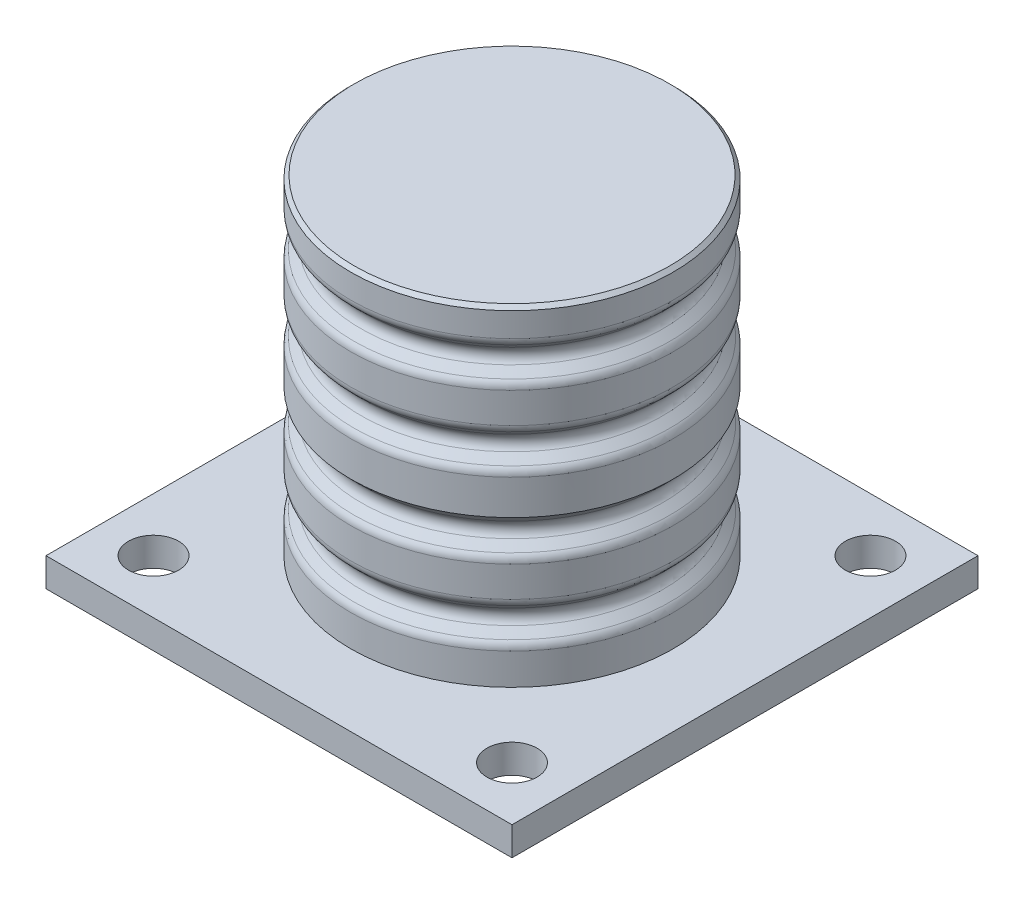
from build123d import *

# Parameters (mm, degrees)
SKETCH2_W           = 130
SKETCH2_H           = 130
SKETCH2_R           = 7
BOSS_EXTRUDE1_DEPTH = 8
SKETCH3_R           = 45
BOSS_EXTRUDE2_DEPTH = 100
CHAMFER1_SIZE       = 1
FILLET1_R           = 3


with BuildPart() as part:
    # Sketch2 → Boss-Extrude1 (new body)
    with BuildSketch(Plane(origin=(0, 0, 0), x_dir=(1, 0, 0), z_dir=(0, 1, 0))):
        Rectangle(SKETCH2_W, SKETCH2_H)
        with Locations(Location((-50, -50, 0), (0, 0, 270))):
            Circle(SKETCH2_R, mode=Mode.SUBTRACT)
        with Locations(Location((-50, 50, 0), (0, 0, 270))):
            Circle(SKETCH2_R, mode=Mode.SUBTRACT)
        with Locations(Location((50, 50, 0), (0, 0, 270))):
            Circle(SKETCH2_R, mode=Mode.SUBTRACT)
        with Locations(Location((50, -50, 0), (0, 0, 270))):
            Circle(SKETCH2_R, mode=Mode.SUBTRACT)
    extrude(amount=BOSS_EXTRUDE1_DEPTH)

    # Sketch3 → Boss-Extrude2 (add)
    with BuildSketch(Plane(origin=(0, 0, 0), x_dir=(1, 0, 0), z_dir=(0, 1, 0))):
        with Locations(Location((0, 0, 0), (0, 0, 270))):
            Circle(SKETCH3_R)
    extrude(amount=BOSS_EXTRUDE2_DEPTH)

    # Chamfer1
    chamfer1_edges = [part.edges().sort_by_distance(p)[0] for p in [
        (0, 100, -45),
    ]]
    chamfer(chamfer1_edges, length=CHAMFER1_SIZE)

    # Sketch4 → Cut-Revolve1 (revolve, cut)
    with BuildSketch(Plane.XY, mode=Mode.PRIVATE) as cut_revolve1_sk:
        Polygon((45, 18), (40, 23), (45, 28), align=None)
        Polygon((45, 39), (40, 44), (45, 49), align=None)
        Polygon((45, 60), (40, 65), (45, 70), align=None)
        Polygon((45, 81), (40, 86), (45, 91), align=None)
    revolve(cut_revolve1_sk.sketch.rotate(Axis((0, 0, 0), (0, 1, 0)), 90), axis=Axis((0, 0, 0), (0, 1, 0)), mode=Mode.SUBTRACT)

    # Fillet1
    fillet1_edges = [part.edges().sort_by_distance(p)[0] for p in [
        (-45, 28, 0),
        (-45, 18, 0),
        (0, 23, 40),
        (-45, 39, 0),
        (0, 44, 40),
        (-45, 70, 0),
        (-45, 60, 0),
        (0, 65, 40),
        (-45, 91, 0),
        (-45, 81, 0),
        (0, 86, 40),
    ]]
    fillet(fillet1_edges, radius=FILLET1_R)


solid = part.part
